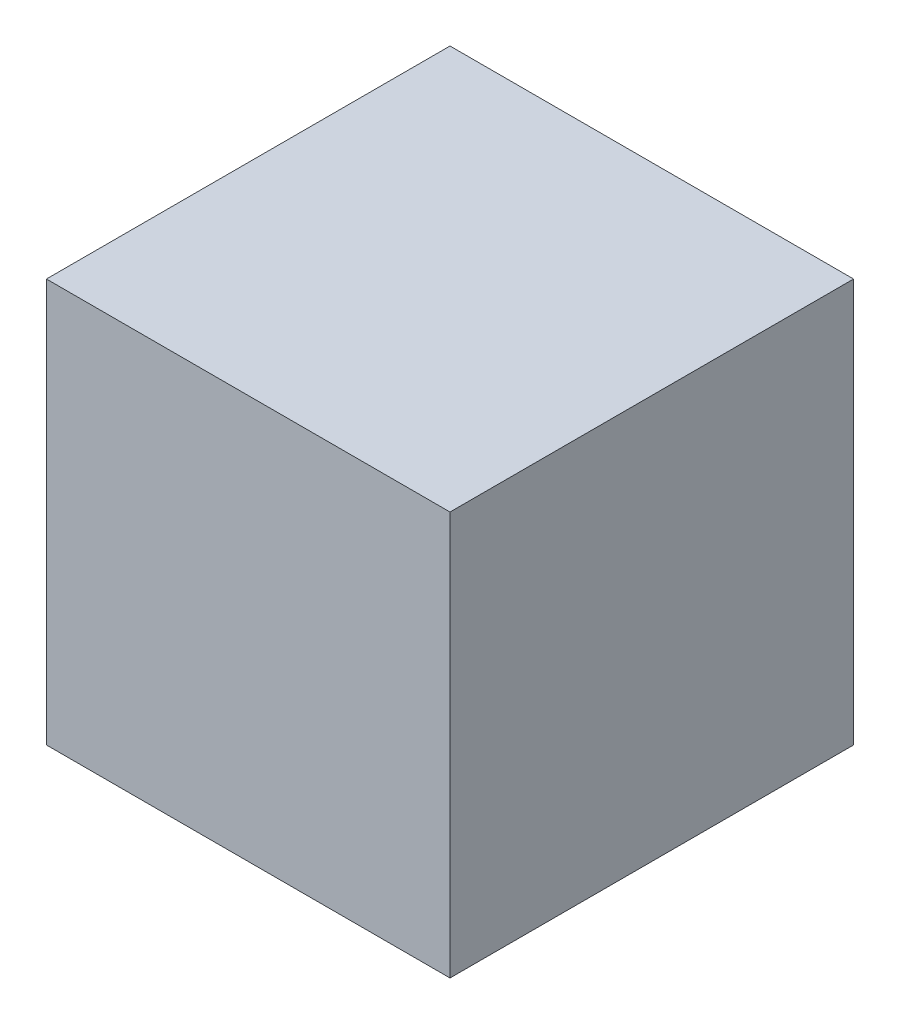
SolidWorks part; units mm, degrees
ref_plane "前视基准面" through (0, 0, 0) normal (0, 0, 1) x (1, 0, 0)
ref_plane "上视基准面" through (0, 0, 0) normal (0, 1, 0) x (1, 0, 0)
ref_plane "右视基准面" through (0, 0, 0) normal (1, 0, 0) x (0, 0, -1)
sketch "草图1" plane through (0, 0, 0) normal (0, 0, 1) x (1, 0, 0)
  line L1 (40, -40) -> (-40, -40)
  line L2 (40, -40) -> (40, 40)
  line L3 (40, 40) -> (-40, 40)
  line L4 (-40, -40) -> (-40, 40)
  line L5 (40, -40) -> (-40, 40) construction
  line L6 (40, 40) -> (-40, -40) construction
  point P0 (0, 0)
  dimension "D1" = 80
extrude "凸台-拉伸1" add sketch "草图1" along normal blind 80
